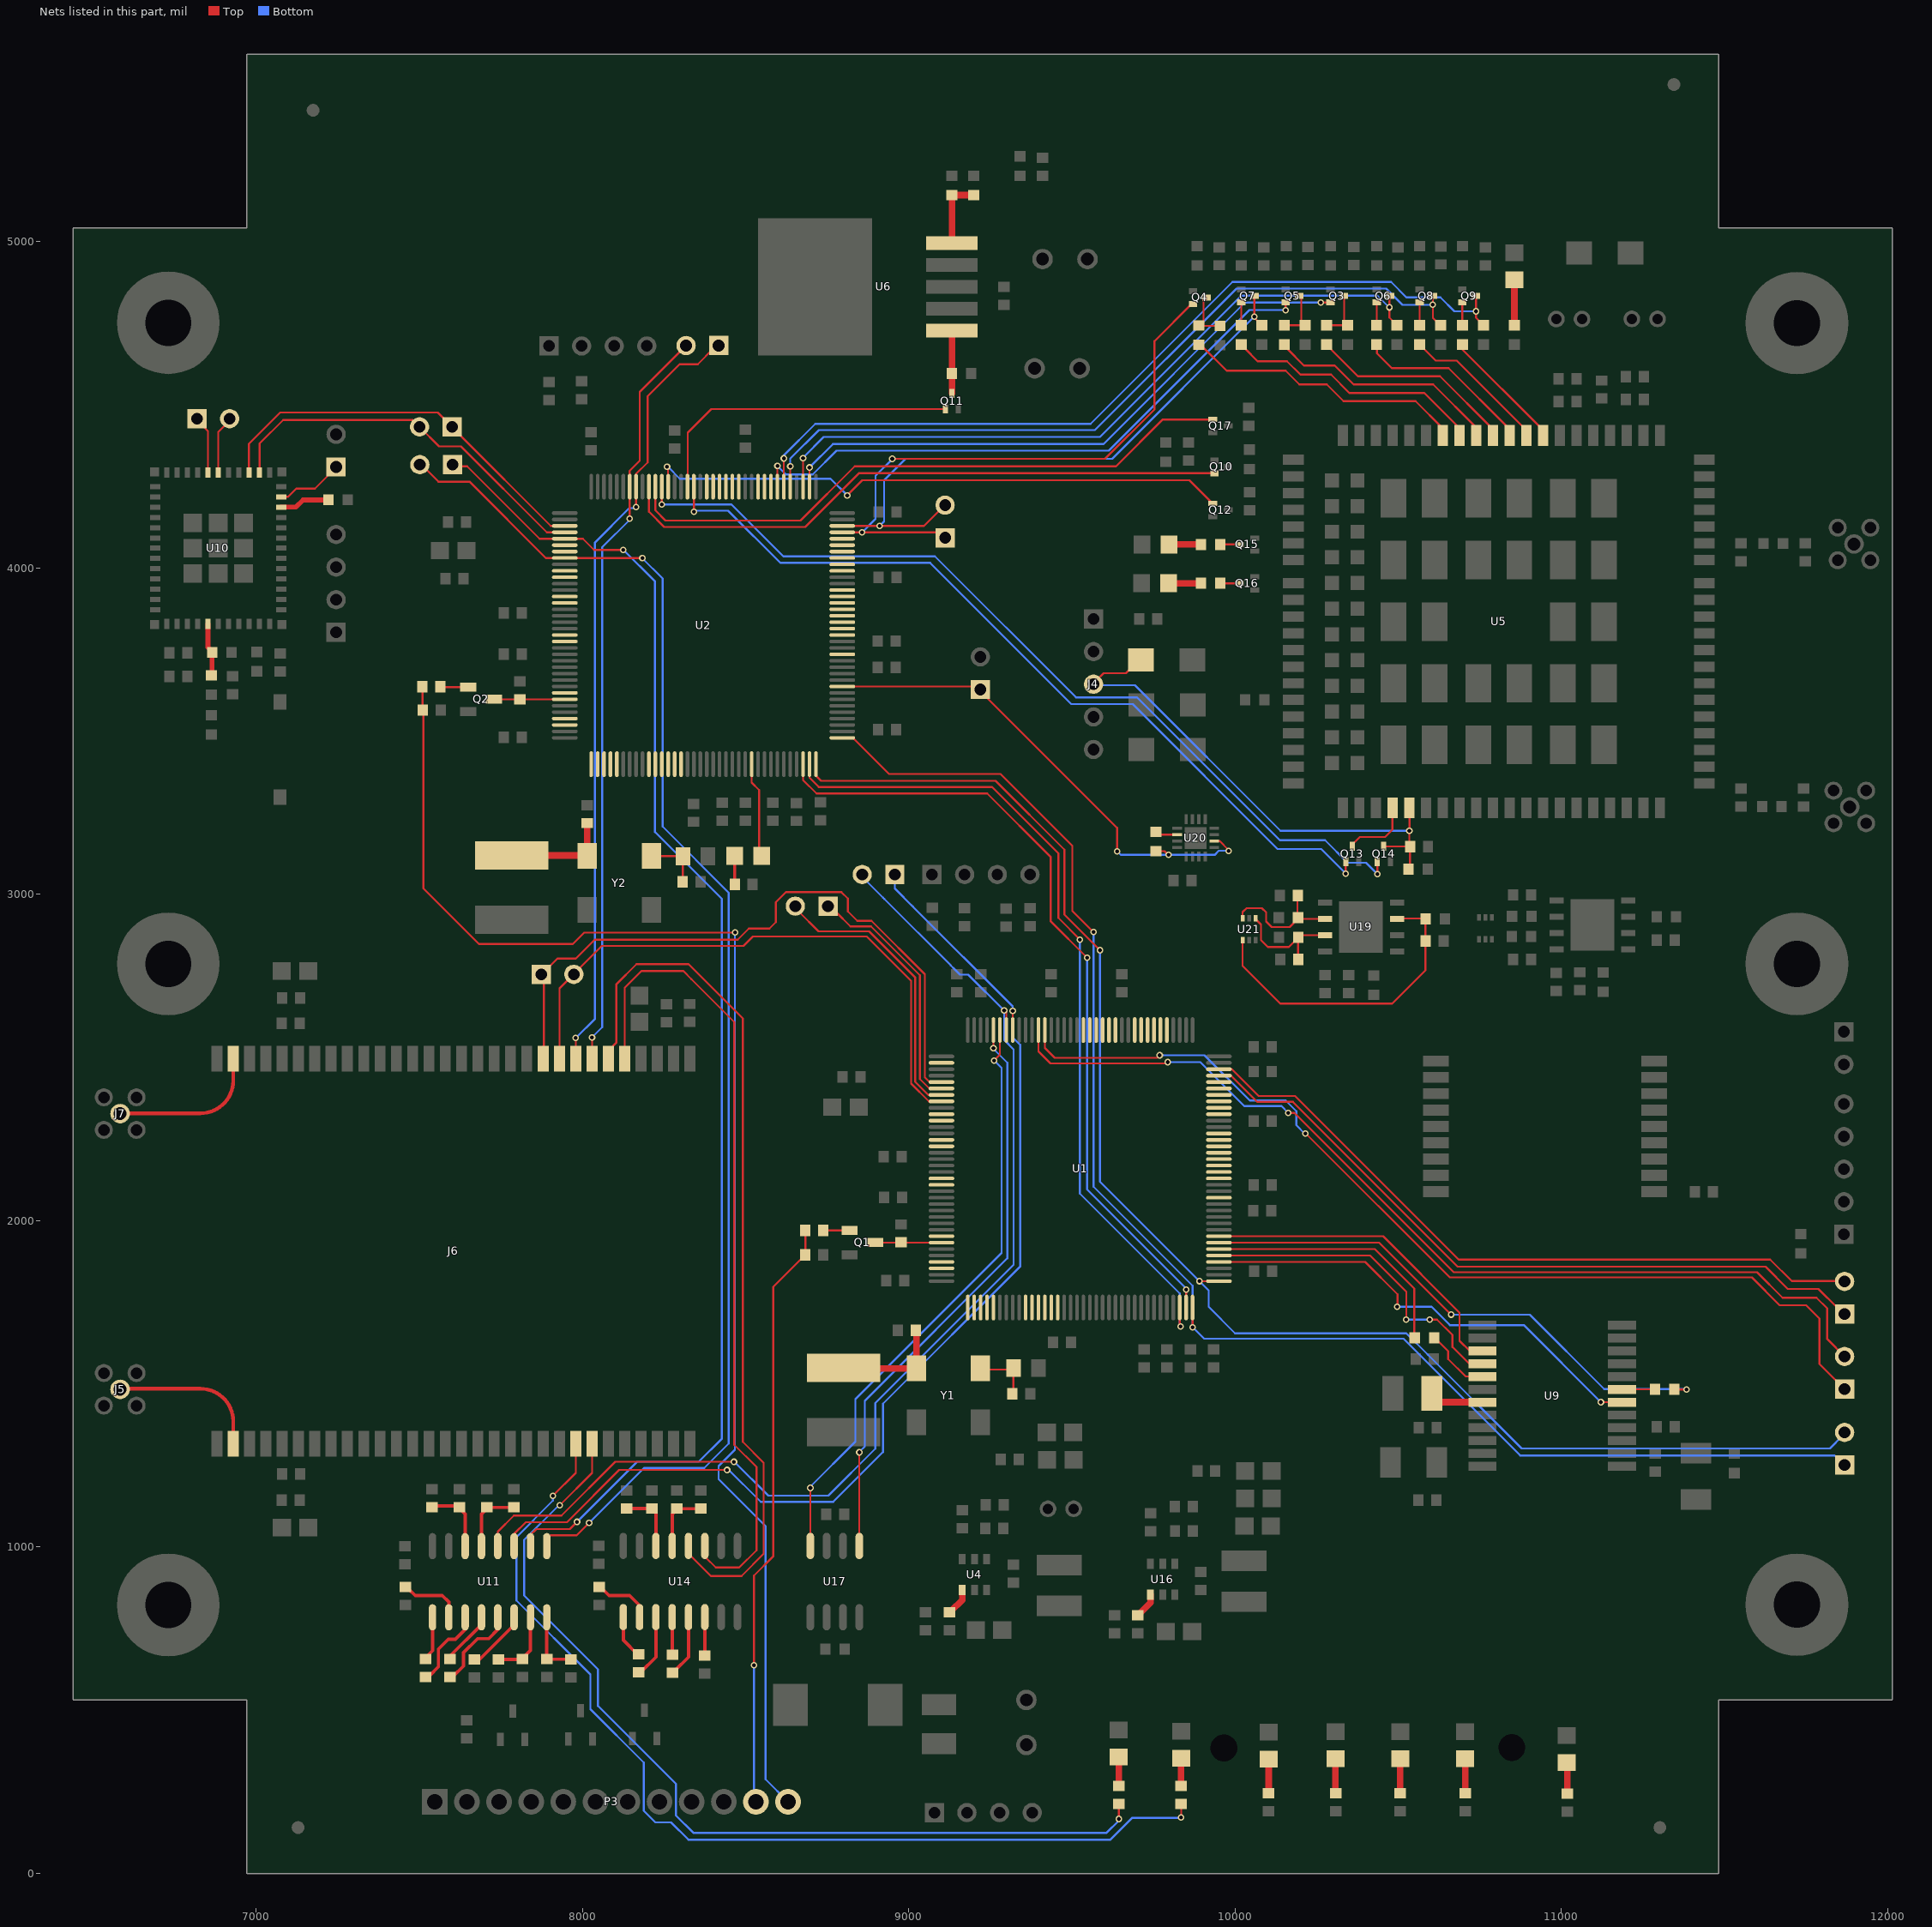
[diagram p0: the nets of this part, all layers, seen from the top]
# Altium PCB MISC86294.PcbDoc (part 6 of 8)
Units mil, origin at the board's own origin, x right, y up, seen from the top; angles counter-clockwise.
Board outline 5574.84 x 5574.84 mil, 4 copper layers (Top, GND02, PWR03, Bottom), stack 23.756 mil thick; 313 components, 311 nets, 1350 pads, 1701 vias.

## Via types
v1: diameter 20, hole 12, Top to Bottom, 1701 vias

## Nets (pads, with @x,y where several pads share a name; then routed paths per layer and width w, separated by ;. In a path a pad name is that pad's centre, name@x,y a point inside that pad or via, vN(x,y) a via of type N, cw(c..) or ccw(c..) an arc to the next point about the centre after c; other vN are vias at no path point) (continued)
NetC106_1: C106.1 U11.3 | length 235
  Top w10: C106.1@7532,607 7558,633 7558,687 7588,717 7610,717 7640.02,747.02 U11.3@7640.02,784.35
NetC106_2: C106.2 U11.1 | length 129.2
  Top w10: C106.2@7521,663 7540.02,682.02 U11.1@7540.02,784.35
NetC108_1: C108.1 U11.5 | length 255.2
  Top w10: C108.1@7605,605 7635,635 7635,676 7678,719 7712,719 7740.02,747.02 U11.5@7740.02,784.35
NetC108_2: C108.2 U11.4 | length 159.5
  Top w10: C108.2@7593,665 7690.02,762.02 U11.4@7690.02,784.35
NetC109_1: C109.1 U14.3 | length 187
  Top w10: C109.1@8179,617 8224.68,662.68 U14.3@8224.68,785.13
NetC109_2: C109.2 U14.1 | length 133.5
  Top w10: U14.1@8124.68,785.13 8124.68,714.32 C109.2@8169,670
NetC110_1: C110.1 U11.2 | length 186.2
  Top w10: C110.1@7467,871 7487,851 7570,851 7590.02,830.98 U11.2@7590.02,784.35
NetC112_1: C112.1 U14.2 | length 165.6
  Top w10: C112.1@8064,868 8081,851 8144,851 8174.68,820.32 U14.2@8174.68,785.13
NetC113_1: C113.1 U11.6 | length 185.3
  Top w10: C113.1@7672,655 7684,655 7790.02,761.02 U11.6@7790.02,784.35
NetC114_1: C114.1 U14.5 | length 180
  Top w10: C114.1@8284,622 8324.68,662.68 U14.5@8324.68,785.13
NetC114_2: C114.2 U14.4 | length 110.4
  Top w10: C114.2@8274.68,674.68 U14.4@8274.68,785.13
NetC115_2: C115.2 R75.2 U11.14 | length 206
  Top w10: C115.2@7543,1126 7615,1126 7640.02,1100.98 U11.14@7640.02,1002.38
NetC116_2: C116.2 R77.2 U11.13 | length 201.9
  Top w10: U11.13@7690.02,1002.38 7690.02,1101.02 7710,1121 C116.2@7785,1121
NetC117_1: C117.1 U14.6 | length 112.8
  Top w10: C117.1@8374.68,672.32 U14.6@8374.68,785.13
NetC118_2: C118.2 R76.2 U14.14 | length 200.9
  Top w10: C118.2@8133,1118 8215,1118 8224.68,1108.32 U14.14@8224.68,1003.16
NetC119_2: C119.2 R78.2 U14.13 | length 195.6
  Top w10: U14.13@8274.68,1003.16 8274.68,1100.68 8291,1117 C119.2@8366,1117
NetC120_1: C120.1 R81.2 U11.8 | length 194.2
  Top w10: U11.8@7890.02,784.35 7890.02,663.02 7897.03,656 C120.1@7960,656
NetC121_1: C121.1 R79.2 U11.7 | length 203
  Top w10: C121.1@7750,655 7812,655 7840.02,683.02 U11.7@7840.02,784.35
NetC123_1: C123.1 R82.2 U19.6 U21.3 | length 391.5
  Top w6: U21.3@10023,2928 10023,2946 10035,2958 10082,2958 10095,2945 10095,2917 10112,2900 10167,2900 10193,2926 R82.2@10193,2929 ; C123.1@10191,2990 10191,2934 10199.97,2925.03 U19.6@10275.59,2925.03
NetC129_1: C129.1 R80.2 U19.7 U21.1 | length 346.9
  Top w6: U21.1@10064,2921 U21.1@10065,2920 ; U21.1@10066,2921 10079,2908 10079,2860 10100,2839 10164.54,2839 R80.2@10193,2867.46 ; C129.1@10193,2812 R80.2@10193,2867.46 ; R80.2@10193.98,2868.45 R80.2@10193,2867.46 ; U19.7@10275.59,2875.03 10197.03,2875.03 10193,2871 R80.2@10193,2867.46
NetC130_1: C130.1 R90.2 U19.3 U21.4 | length 958
  Top w6: U21.4@10023,2861 10023,2781 10138.5,2665.5 10456.17,2665.5 10481.5,2665.5 10583.42,2767.42 C130.1@10583.42,2856.97 10583.42,2918.42 10575.84,2926 U19.3@10510,2926
NetC200_2: C200.2 R200.2 Y1.3 | length 193.7
  Top w6: Y1.3@9217.02,1543.84 R200.2@9324.84,1543.84 ; C200.2@9319.98,1456.16 R200.2@9319.98,1542.03
NetC201_1: C201.1 L200.1 Y1.4 | length 246.2
  Top w20: L200.1@8889,1548 8889.84,1547.16 9023.16,1547.16 C201.1@9023.16,1658.9
NetC202_2: C202.2 R201.2 Y2.3 | length 188.1
  Top w6: Y2.3@8211.06,3117.66 R201.2@8306.34,3117.66 ; C202.2@8306.89,3038.29 R201.2@8306.89,3124.11 ; C202.2@8308,3042 C202.2@8312.94,3037.06
NetC203_1: C203.1 L201.1 Y2.4 | length 318.5
  Top w20: L201.1@7782.37,3119.29 Y2.4@8010.29,3119.29 ; Y2.4@8014.05,3127.95 C203.1@8014.05,3218.57
NetD2_1: D2.1 R32.1 | length 74.9
  Top w20: R32.1@11017.89,244.25 D2.1@11017.89,319.11
NetD3_1: D3.1 R92.2 | length 78.6
  Top w20: R92.2@9834.65,267.73 D3.1@9834.65,346.35
NetD8_2: D8.2 R64.1 | length 131.5
  Top w20: R64.1@10856.07,4744.45 D8.2@10856.07,4875.93
NetD9_2: D9.2 R65.1 | length 100.4
  Top w20: D9.2@9794.52,4072.48 R65.1@9894.96,4072.48
NetD10_2: D10.2 R66.1 | length 78.1
  Top w20: D10.2@9810.52,3953.48 R66.1@9888.59,3953.48
NetD11_1: D11.1 R93.2 | length 86.4
  Top w20: D11.1@9636,351 9643.65,343.35 R93.2@9643.65,267.73
NetD12_1: D12.1 R84.2 | length 77
  Top w10: R84.2@8466.14,3030.11 D12.1@8466.14,3107.14
NetD12_2: D12.2 U2.26 | length 291.6
  Top w6: U2.26@8518.25,3399.13 8518.25,3342.75 8541,3320 D12.2@8541,3117
NetD13_1: D13.1 R7.2 | length 99.1
  Top w20: R7.2@10307.52,251.48 D13.1@10307.52,350.59
NetD14_1: D14.1 R6.2 | length 97.3
  Top w20: R6.2@10103,253 D14.1@10103,350.3
NetD15_1: D15.1 R9.2 | length 101.6
  Top w20: R9.2@10505.96,249.04 D15.1@10505.96,350.59
NetD16_1: D16.1 R98.2 | length 101.5
  Top w20: R98.2@10705.04,249.04 D16.1@10705.04,350.59
NetJ5_1: J5.1 J6.2 | length 460.3
  Top w11.55: J5.1@6595,1485 6829.01,1485 cw(c6829.01,1385) 6929.01,1385 J6.2@6929.01,1315.83
NetJ6_23: J6.23 R92.1 | length 3113.3
  Top w6: v1(7909,1157) 7979.01,1227.01 J6.23@7979.01,1315.83 ; v1(9834.65,170.65) R92.1@9834.65,212.62
  Bottom w6: v1(7909,1157) 7909,1142 7797,1030 7797,836 8024,609 8024,503 8187.64,339.36 8187.64,191.36 8223,156 8271,156 8324,103 9618,103 9685,170 v1@9833,170
NetJ6_24: J6.24 R93.1 | length 2860.9
  Top w6: v1(7930,1128) 8029.01,1227.01 J6.24@8029.01,1315.83 ; v1(9643.65,166.35) R93.1@9643.65,212.62
  Bottom w6: v1@7927,1128 7820.5,1021.5 7820.5,851.5 8047,625 8047,513 8286,274 8286,177 8339,124 9606,124 v1@9644,162 ; v1@7928.5,1126.5 v1(7930,1128)
NetJ6_35: J6.35 U14.11 | length 2476.8
  Top w6: J6.35@8129.01,2496.94 8129.01,2696 8129,2714 8180,2765 8309,2765 8333.5,2740.5 8465,2609 8465,1313 8533,1245 8533,990 8480,937 8408,937 U14.11@8377,968
NetJ6_36: J6.36 U14.12 | length 2695.9
  Top w6: J6.36@8079.01,2496.94 J6.36@8079.01,2525 ; J6.36@8083,2525 8103,2545 8103,2724 8165,2786 8325,2786 8351,2760 8491,2620 8491,1322 8555,1258 8555,979 8487,911 8393,911 8324.68,979.32 U14.12@8324.68,1003.16
NetJ6_37: J6.37 J15.2 U2.102 | length 2283.8
  Top w6: J6.37@8029.01,2496.94 v1(8029.01,2560.99) ; v1(8144.23,4151.23) U2.102@8144.23,4249.52 8144.23,4298.23 8175,4329 8175,4540 J15.2@8305,4670
  Bottom w6: v1(8029.01,2560.99) v1@8030.51,2562.49 ; v1@8030,2563 8060,2593 8060,4064 v1@8144,4148
NetJ6_38: J6.38 J15.1 U2.101 | length 2391.5
  Top w6: J6.38@7979.01,2496.94 v1(7979.01,2559.99) ; v1(8163.92,4187.08) U2.101@8163.92,4249.52 8163.92,4288.92 8199,4324 8199,4527 8297,4625 8353,4625 J15.1@8400,4672
  Bottom w6: v1(7979.01,2559.99) 8038,2618.97 8038,4009 8038,4079 8143,4184 v1@8164,4184
NetJ6_39: J6.39 J20.2 U1.116 | length 1845.6
  Top w6: J6.39@7929.01,2496.94 7929.01,2521 7929,2712 8059,2842 8215,2842 8493,2842 8522,2871 8871,2871 9007,2735 9007,2420 9061.31,2365.69 U1.116@9099.8,2365.69
NetJ6_40: J6.40 J20.1 U1.113 | length 2044.4
  Top w6: J6.40@7880,2521 J6.40@7880,2536 ; J20.1@7880,2760 7923,2803 7979,2803 8037,2861 8197,2861 8475,2861 8509.5,2895.5 8572.5,2895.5 8592,2915 8592,2976 8623,3007 8793,3007 8813,2987 8813,2948 8842,2919 8885,2919 9049,2755 9049,2439 9063.25,2424.75 U1.113@9099.8,2424.75 ; J6.40@7881,2536 7881,2755 7881,2757 J20.1@7882,2758
NetJ6_59: J6.59 J7.1 | length 458
  Top w11.55: J7.1@6596,2329 6829.01,2329 ccw(c6829.01,2429) 6929.01,2429 J6.59@6929.01,2496.94
NetJ9_1: J9.1 U10.23 | length 175.5
  Top w6: U10.23@7075.91,4218.48 7097.48,4218.48 7122.5,4243.5 7179.5,4243.5 J9.1@7223,4287
NetJ10_1: J10.1 U10.31 | length 167.9
  Top w6: J10.1@6822,4449 6851.5,4419.5 U10.31@6851.5,4293.28
NetJ10_2: J10.2 U10.30 | length 164.7
  Top w6: U10.30@6883,4293.28 6883,4417 J10.2@6912,4446
NetJ12_1: J12.1 U1.114 | length 733.1
  Top w6: J12.1@8777,2946 8821,2902 8884,2902 9034,2752 9034,2434 9062.94,2405.06 U1.114@9099.8,2405.06
NetJ12_2: J12.2 U1.115 | length 861.3
  Top w6: J12.2@8662,2948 8723,2887 8878,2887 9019,2746 9019,2717 ; 9019,2720 9019,2717 ; U1.115@9099.8,2385.38 9059.62,2385.38 9019,2426 9019,2717
NetJ13_1: J13.1 U1.101 U11.11 | length 3517
  Top w6: U11.11@7790.02,1002.38 7790.02,1040.02 7826,1076 7952,1076 8112,1236 v1(8443,1236) ; U1.101@9318.31,2584.2 v1(9318.31,2643.31)
  Bottom w6: v1@8443,1241 8546,1138 8768,1138 8921,1291 8921,1439 9341,1859 9341,2539 9318.31,2561.69 v1(9318.31,2643.31) 9318.31,2656.69 9013,2962 ; J13.1@8957,3053 8957,3018 9013,2962 ; 9008,2967 9013,2962
NetJ13_2: J13.2 U1.102 U11.12 | length 3609.8
  Top w6: U11.12@7740.02,1002.38 7740.02,1047.02 7789,1096 7935,1096 8100,1261 v1@8463,1261 ; v1@8465,1259 v1@8463,1261 ; v1@8465,1261 v1(8464,1261) v1@8463,1261 ; v1(9292,2644) 9298.24,2644 9298.62,2643.62 U1.102@9298.62,2584.2
  Bottom w6: v1@8465,1261 8569,1157 8753,1157 8897,1301 8897,1441 9321,1865 9321,2525 9292,2554 v1(9292,2644) 9182,2754 9157,2754 9139.7,2771.3 9139.43,2771.3 9128.3,2782.43 9128.3,2782.7 8925,2986 ; J13.2@8848,3048 8863,3048 8925,2986 ; 8921,2990 8925,2986
NetJ14_1: J14.1 U1.36 U2.37 | length 4686.6
  Top w6: U2.37@8799,3479.84 U2.37@8795.81,3479.84 8828.16,3479.84 8939,3369 9281,3369 9501,3149 9501,2949 v1@9566.5,2883.5 ; v1(9869.49,1673.49) U1.36@9869.49,1733.8
  Bottom w6: 9566,2781 9566,2776 ; v1(9566,2885) 9566,2776 ; J14.1@11848,1269 11837,1280 10874,1280 10516,1638 9904.98,1638 v1(9869.49,1673.49) 9869.49,1800.51 9566,2104 9566,2776
NetJ14_2: J14.2 U1.37 U2.36 | length 4699.2
  Top w6: U2.36@8715.1,3399.13 8715.1,3363.9 8731,3348 8802,3348 ; 8824,3348 8802,3348 ; v1(9586,2829) 9477,2938 9477,3137 9266,3348 8802,3348 ; v1(9890.49,1814.51) U1.37@9950.2,1814.51
  Bottom w6: v1@9586,2826 9586,2119 v1(9890.49,1814.51) 9919,1786 9919,1736 10000,1655 10525,1655 10590,1590 ; 10593,1587 10590,1590 ; 11628,1302 11623,1302 ; J14.2@11860,1339 11823,1302 11623,1302 ; 10590,1590 10878,1302 11623,1302
NetJ16_1: J16.1 U1.69 | length 2226.6
  Top w6: U1.69@9950.2,2444.43 9987.57,2444.43 10068,2364 10177,2364 10519.5,2021.5 ; 10546,1995 10519.5,2021.5 ; J16.1@11845,1734 11788,1791 11694,1791 11626,1859 10682,1859 10519.5,2021.5
NetJ16_2: J16.2 U1.70 | length 2181.7
  Top w6: U1.70@9950.2,2464.12 9989.88,2464.12 10072,2382 10184,2382 10685,1881 11640,1881 11706,1815 J16.2@11863,1815
NetJ17_1: J17.1 Q4.1 U2.69 | length 1809.5
  Top w6: U2.69@8795.81,4109.76 v1(8856.76,4109.76) J17.1@9097.24,4109.76 ; v1(8949,4335) 9601,4335 9753,4487 9753,4696 9868,4811 Q4.1@9874,4811
  Bottom w6: v1(8856.76,4109.76) 8898,4151 8898,4283 v1@8949,4334 ; v1@8952,4331 v1@8952,4332
NetJ17_2: J17.2 Q7.3 R44.1 U2.70 | length 1900.5
  Top w6: U2.70@8795.81,4129.44 v1(8910.44,4129.44) 9046.44,4129.44 J17.2@9096,4179 ; v1@10059,4767.55 R44.1@10082.1,4744.45 ; v1(10059,4771) Q7.3@10059,4830
  Bottom w6: v1(8910.44,4129.44) 8924,4143 8924,4269 8990,4335 9623,4335 v1(10059,4771)
NetJ19_1: J19.1 U2.111 U10.27 | length 1235.4
  Top w6: U10.27@6977,4298 6977,4381 7073,4477 7556,4477 J19.1@7600,4433 J19.1@7622.5,4410.5 ; J19.1@7622,4410 7902.56,4129.44 U2.111@7945.42,4129.44
NetJ19_2: J19.2 U2.112 U10.26 | length 1189.8
  Top w6: U10.26@7010,4300 7010,4382 7082,4454 7479,4454 J19.2@7500,4433 7560,4373 7627,4373 7890.24,4109.76 U2.112@7945.42,4109.76
NetJ21_1: J21.1 U2.113 U11.10 | length 4221.4
  Top w6: J21.1@7603,4312 7646,4312 7867.93,4090.07 U2.113@7945.42,4090.07 8000.93,4090.07 8035,4056 v1(8124,4056) ; U11.10@7840.02,1002.38 7840.02,1037.02 7858,1055 7961,1055 v1(7983,1077)
  Bottom w6: v1(7983,1077) 8167,1261 8356,1261 8427,1332 8427,2986 8222,3191 8222,3959 v1@8124,4057
NetJ21_2: J21.2 U2.116 U11.9 | length 4327.3
  Top w6: J21.2@7515,4308 7558,4265 7653,4265 7886.98,4031.02 U2.116@7945.42,4031.02 v1(8183.02,4031.02) ; U11.9@7890.02,1002.38 7890.02,1024.02 7902,1036 7982,1036 v1(8020,1074)
  Bottom w6: v1(8020,1074) 8188,1242 8373,1242 8448,1317 8448,2909 ; v1@8181,4032 8245,3968 8245,3459 ; 8245,3470 8245,3459 ; 8448,2916 8448,2909 ; 8245,3459 8245,3208 8448,3005 8448,2909
NetJ22_1: J22.1 U1.96 | length 3051.9
  Top w6: U1.96@9416.73,2584.2 9416.73,2529.27 9447,2499 9761,2499 v1(9769,2507) ; v1@10215.5,2268.5 10658,1826 11584,1826 11669,1741 11750,1741 11791,1700 11791,1561 J22.1@11868,1484
  Bottom w6: v1(9769,2507) 9906,2507 10045,2368 10155,2368 10187.5,2335.5 10187.5,2292.5 v1@10214,2266
  other v1: 10215,2267
NetJ22_2: J22.2 U1.97 | length 2981.2
  Top w6: U1.97@9397.05,2584.2 9397.05,2518.95 9434,2482 v1@9789,2482 ; v1@10158,2330 v1(10163,2330) 10182,2330 10670,1842 11600,1842 11678,1764 11782,1764 11815,1731 11815,1637 J22.2@11868,1584
  Bottom w6: v1(9793,2486) 9893,2486 10028,2351 10142,2351 v1(10163,2330)
NetJ23_1: J23.1 R91.1 U2.45 U20.2 | length 1563.6
  Top w6: U2.45@8795.81,3637.32 9204.68,3637.32 9638,3204 v1(9638,3132) ; R91.1@9756.87,3132.36 9783.64,3132.36 v1@9795,3121 ; U20.2@9936.24,3163.25 9952.75,3163.25 v1@9979,3137 ; v1(9980,3133) 9980,3128 9981,3128 9981,3138 v1@9980.5,3138.5
  Bottom w6: v1@9638,3133 9650,3121 v1(9796,3121) 9937,3121 9950,3134 v1@9979,3134 ; v1@9979,3132 9978,3131 9980,3131 v1(9980,3133)
NetL2_2: L2.2 U9.7 | length 128.8
  Top w20: L2.2@10629.27,1443.73 U9.7@10758.02,1443.73
NetP3_11: P3.11 R1.1 R2.2 | length 1784
  Top w6: v1(8525,638) 8525,912 8584,971 8584,1796.39 R1.1@8682.5,1894.89 ; R1.1@8682.89,1904.11 R2.2@8682.89,1970
  Bottom w6: P3.11@8525,242 v1(8525,638)
NetP3_12: P3.12 R13.1 R14.2 | length 4420.5
  Top w6: R13.1@7509.14,3575.14 R14.2@7509.14,3635.95 ; R13.1@7512,3562 7512,3018 7682,2848 7970,2848 8005,2883 v1(8467,2883)
  Bottom w6: v1@8467,2886 v1(8467,2883) 8467,1298 8417,1248 8417,1208 8561,1064 8561,287.76 P3.12@8629.71,219.05
NetQ1_1: Q1.1 R2.1 | length 73.2
  Top w6: R2.1@8745.4,1970.4 Q1.1@8818.63,1970.4
NetQ1_3: Q1.3 R3.2 U1.138 | length 194.2
  Top w6: Q1.3@8905.62,1932.62 U1.138@9099.8,1932.62
NetQ2_1: Q2.1 R14.1 | length 77.1
  Top w6: R14.1@7572.32,3635.32 Q2.1@7649.44,3635.32
NetQ2_3: Q2.3 R16.2 U2.138 | length 208.5
  Top w6: Q2.3@7736.95,3597.95 U2.138@7945.42,3597.95
NetQ3_1: Q3.1 U2.74 | length 1862.4
  Top w6: U2.74@8695.42,4249.52 v1(8695.42,4308.59) ; v1(10263,4814) 10288,4814 Q3.1@10289,4813
  Bottom w6: v1(8695.42,4308.59) 8766.83,4380 9596,4380 10030,4814 v1(10263,4814)
NetQ3_3: Q3.3 R37.2 R41.1 | length 144.7
  Top w6: R41.1@10280.6,4744.45 R37.2@10333.45,4744.45 ; Q3.3@10334,4832 10334,4754.95 R37.2@10344.5,4744.45
NetQ4_3: Q4.3 R39.2 R53.1 | length 142.4
  Top w6: R53.1@9896.45,4742.45 R39.2@9953.8,4742.45 ; R53.1@9903,4748 9903,4825 9903,4826 Q4.3@9908,4831
NetQ5_1: Q5.1 U2.79 | length 1864.2
  Top w6: U2.79@8596.99,4249.52 v1(8596.99,4312.99) ; v1(10154.78,4790.22) Q5.1@10154.78,4814.45
  Bottom w6: v1(8596.99,4312.99) 8622.98,4287 8705,4287 8778,4360 9613,4360 10044,4791 v1@10154,4791
NetQ5_3: Q5.3 R40.2 R48.1 | length 142.2
  Top w6: R48.1@10161.55,4744.45 R40.2@10214.45,4744.45 10203,4755.9 Q5.3@10203,4829
NetQ6_1: Q6.1 R43.1 | length 63.2
  Top w6: R43.1@10434.24,4751.24 Q6.1@10434.24,4814.45
NetQ6_3: Q6.3 R42.1 U2.75 | length 2202.6
  Top w6: U2.75@8675.73,4249.52 v1(8675.73,4336.73) ; Q6.3@10473,4832 v1(10473,4799) 10473,4767.75 R42.1@10496.3,4744.45
  Bottom w6: v1(8675.73,4336.73) v1@8678,4336.73 ; v1@8678,4341 8739,4402 9586,4402 10019,4835 10436,4835 10473,4798 v1(10473,4799)
NetQ7_1: Q7.1 R51.1 | length 64.8
  Top w6: R51.1@10018.62,4749.62 Q7.1@10018.62,4814.45
NetQ8_1: Q8.1 R47.1 | length 60
  Top w6: R47.1@10565.41,4754.41 Q8.1@10565.41,4814.45
NetQ8_3: Q8.3 R52.1 U2.77 | length 2388.1
  Top w6: U2.77@8636.36,4249.52 v1(8636.36,4311.64) ; Q8.3@10606,4830 v1(10606,4807) 10606,4767 10628.55,4744.45 R52.1@10630.09,4744.45
  Bottom w6: v1(8636.36,4311.64) 8636.36,4335.36 8724,4423 9570,4423 10004,4857 10463,4857 10513,4807 v1@10604,4807 ; v1@10605,4808 v1(10606,4807)
NetQ9_1: Q9.1 R50.1 | length 66
  Top w6: R50.1@10696.59,4748.41 Q9.1@10696.59,4814.45
NetQ9_3: Q9.3 R55.1 U2.78 | length 2570.9
  Top w6: U2.78@8616.67,4249.52 v1(8616.67,4336.32) ; Q9.3@10738,4831 v1(10738,4787) 10738,4767.34 R55.1@10760.89,4744.45
  Bottom w6: v1(8616.67,4336.32) 8616.67,4345.68 8713,4442 9557,4442 9992,4877 10478,4877 10525,4830 10629,4830 10672,4787 v1(10738,4787)
NetQ10_1: Q10.1 U2.99 | length 1865.5
  Top w6: U2.99@8203,4217 8203,4173 8250,4126 8682,4126 8846.6,4290.6 Q10.1@9936.82,4290.6
NetQ11_1: Q11.1 U2.93 | length 980.2
  Top w6: U2.93@8322,4255 8322,4415 8394.7,4487.7 Q11.1@9112.04,4487.7
NetQ11_3: Q11.3 R59.1 U6.1 | length 183
  Top w20: Q11.3@9132.04,4534.95 U6.1@9132.04,4717.96
NetQ12_1: Q12.1 U2.96 | length 1798.2
  Top w6: v1(8259,4311) 8261,4311 8262,4310 U2.96@8262,4280 ; v1(8811,4223) 8857,4269 9859.98,4269 Q12.1@9930.93,4198.05 Q12.1@9922.95,4198.05
  Bottom w6: v1(8259,4311) 8261,4311 8298,4274 8760,4274 v1(8811,4223)
NetQ13_1: Q13.1 U2.92 | length 2569
  Top w6: v1(8341.08,4172.92) U2.92@8341.08,4249.52 ; v1(10338.92,3063.08) Q13.1@10338.92,3099.74
  Bottom w6: v1@8341,4176 8446,4176 8606,4016 9065,4016 9498,3583 9686,3583 10130,3139 10264,3139 v1@10337,3066
NetQ14_1: Q14.1 U2.97 | length 2748.1
  Top w6: v1(8242.66,4195.34) U2.97@8242.66,4249.52 ; v1(10435.68,3062.32) Q14.1@10435.68,3099.74
  Bottom w6: v1@8246,4195 8456,4195 8615,4036 9080,4036 9512,3604 9699,3604 10137,3166 10276,3166 10345,3097 10401,3097 v1@10434,3064
NetQ15_3: Q15.3 R65.2 | length 48
  Top w6: R65.2@9965.48,4072.48 Q15.3@10013.49,4072.48
NetQ16_3: Q16.3 R66.2 | length 58
  Top w6: R66.2@9955.48,3953.48 Q16.3@10013.49,3953.48
NetQ17_1: Q17.1 U2.98 | length 1893
  Top w6: U2.98@8223,4220 8223,4177 8254,4146 8668,4146 8834,4312 9635,4312 9778.6,4455.6 Q17.1@9931.93,4455.6
NetR23_1: R23.1 U1.43 | length 1656
  Top w6: U1.43@9950.2,1932.62 10441.38,1932.62 v1(10662,1712) v1@10662.5,1711.5 ; R23.1@11346.64,1482.87 v1(11383.13,1482.87)
  Bottom w6: v1(10662,1712) 10768,1712 10903,1712 11131,1484 v1@11380,1484 ; v1@11380,1482.87 v1(11383.13,1482.87)
NetR23_2: R23.2 U9.19 | length 90.9
  Top w6: U9.19@11185.98,1483.1 R23.2@11276.9,1483.1
NetR24_1: R24.1 U1.42 | length 788.9
  Top w6: U1.42@9950.2,1912.94 10428.06,1912.94 10549,1792 R24.1@10549,1652
NetR24_2: R24.2 U9.5 | length 199.3
  Top w6: R24.2@10619,1634 10653,1600 10653,1576 10706.53,1522.47 U9.5@10758.02,1522.47
NetR26_1: R26.1 U4.4 | length 77.7
  Top w20: R26.1@9130,804 9163.6,837.6 U4.4@9163.6,867.76
NetR30_1: R30.1 U16.4 | length 74.5
  Top w20: R30.1@9705,794 9740.6,829.6 U16.4@9740.6,853.76
NetR41_2: R41.2 U5.65 | length 624.8
  Top w6: R41.2@10288,4676 10376,4588 10628,4588 10790.28,4425.72 U5.65@10790.28,4406.86
NetR43_2: R43.2 U5.64 | length 538.4
  Top w6: R43.2@10435,4675 10435,4658 10480,4613 10654,4613 10841.46,4425.54 U5.64@10841.46,4406.86
NetR47_2: R47.2 U5.63 | length 434
  Top w6: R47.2@10578,4673 10615,4636 10679,4636 10892.64,4422.36 U5.63@10892.64,4406.86
NetR48_2: R48.2 U5.66 | length 705.8
  Top w6: R48.2@10158,4674 10211,4621 10305,4621 10363,4563 10607,4563 10739.1,4430.9 U5.66@10739.1,4406.86
NetR50_2: R50.2 U5.62 | length 377.3
  Top w6: R50.2@10690,4679 10690,4677 10943.82,4423.18 U5.62@10943.82,4406.86
NetR51_2: R51.2 U5.67 | length 782.6
  Top w6: R51.2@10029,4674 10069,4634 10159,4634 10200,4593 10294,4593 10350,4537 10580,4537 10687.92,4429.08 U5.67@10687.92,4406.86
NetR53_2: R53.2 U5.68 | length 864.8
  Top w6: R53.2@9897,4680 R53.2@9901,4676 ; R53.2@9902,4677 9974,4605 10155,4605 10197,4563 10281,4563 10332,4512 10553,4512 10636.74,4428.26 U5.68@10636.74,4406.86
NetR60_1: R60.1 R63.2 U6.5 | length 200
  Top w20: U6.5@9132.17,5006.17 R63.2@9132.17,5143.17 R60.1@9195.17,5143.17
NetR71_1: R71.1 R72.1 U10.5 | length 154.9
  Top w15: U10.5@6851.5,3828.72 6851.5,3757.5 6864,3745 R71.1@6864,3679
NetR74_2: R74.2 U10.22 | length 148.2
  Top w15: U10.22@7075.91,4186.98 7120.98,4186.98 7143,4209 R74.2@7215,4209
NetR91_2: R91.2 U20.10 | length 50.9
  Top w6: R91.2@9771.13,3182.87 U20.10@9822.07,3182.87
NetU1_1: U1.1
NetU1_2: U1.2
NetU1_3: U1.3
NetU1_4: U1.4
NetU1_5: U1.5
NetU1_10: U1.10
NetU1_11: U1.11
NetU1_12: U1.12
NetU1_13: U1.13
NetU1_14: U1.14
NetU1_15: U1.15
NetU1_34: U1.34 U2.35 | length 2569.4
  Top w6: U2.35@8695.42,3399.13 8695.42,3357.59 8724,3329 9255,3329 9458,3126 9458,2928 v1@9526,2860 ; U1.34@9830.12,1733.8 9830.12,1676.12 9830.24,1676 v1(9833,1676)
  Bottom w6: v1(9524,2861) 9524,2774 9524,2083 9830.12,1776.88 9830.12,1676.12 9830.24,1676 v1(9833,1676)
NetU1_35: U1.35 U2.34 | length 2461.2
  Top w6: U2.34@8675.73,3399.13 8675.73,3350.27 8717,3309 8782,3309 ; 8790,3309 8782,3309 ; v1@9545,2807 9435,2917 9435,3114 9240,3309 8782,3309 ; U1.35@9849.8,1733.8 v1(9849.8,1788.8)
  Bottom w6: v1(9546,2806) 9546,2096 v1@9849.8,1792.2
NetU1_40: U1.40 U9.18 | length 1433.9
  Top w6: U1.40@9950.2,1873.57 10398.43,1873.57 10498,1774 v1@10498,1737 ; v1(11121.27,1443.73) U9.18@11185.98,1443.73
  Bottom w6: v1(10496,1736) 10602,1736 10658,1680 10885,1680 v1@11119,1446
NetU1_41: U1.41 U9.4 | length 1018.6
  Top w6: U1.41@9950.2,1893.25 10413.75,1893.25 10525,1782 10525,1742 ; v1@10525,1700 10525,1742 ; 10525,1738 10525,1742 ; v1(10596,1697) 10619,1697 10666,1650 10666,1613 10717.16,1561.84 U9.4@10758.02,1561.84
  Bottom w6: v1(10524,1697) v1(10596,1697)
NetU1_44: U1.44 U9.3 | length 989.7
  Top w6: U1.44@9950.2,1952.31 10453.69,1952.31 10688,1718 10688,1632 10719,1601 U9.3@10744,1601
NetU1_50: U1.50
NetU1_53: U1.53
NetU1_54: U1.54
NetU1_55: U1.55
NetU1_56: U1.56
NetU1_57: U1.57
NetU1_58: U1.58
NetU1_59: U1.59
NetU1_60: U1.60
NetU1_63: U1.63
NetU1_64: U1.64
NetU1_65: U1.65
NetU1_66: U1.66
NetU1_67: U1.67
NetU1_68: U1.68
NetU1_77: U1.77
NetU1_78: U1.78
NetU1_79: U1.79
NetU1_80: U1.80
NetU1_81: U1.81
NetU1_82: U1.82
NetU1_85: U1.85
NetU1_86: U1.86
NetU1_87: U1.87
NetU1_88: U1.88
NetU1_89: U1.89
NetU1_90: U1.90
NetU1_103: U1.103 U17.4 | length 1841.7
  Top w6: U17.4@8698,1003 v1(8698,1181) ; v1(9261,2491) 9278.94,2508.94 U1.103@9278.94,2584.2
  Bottom w6: v1@8696,1181 v1(8698,1181) ; v1@8696,1183 8836,1323 8836,1453 9284,1901 9284,2468 v1(9261,2491)
NetU1_104: U1.104 U17.1 | length 1780.2
  Top w6: U17.1@8848,1003 v1(8848,1290) ; v1(9259.25,2528.25) U1.104@9259.25,2584.2
  Bottom w6: v1@8850,1293 8864.72,1307.72 8864.72,1447.72 9302,1885 9302,2484 v1@9261,2525 ; v1@9260,2528 v1@9261,2528
NetU1_110: U1.110
NetU1_118: U1.118
NetU1_119: U1.119
NetU1_122: U1.122
NetU1_123: U1.123
NetU1_128: U1.128
NetU1_129: U1.129
NetU1_137: U1.137
NetU1_141: U1.141
NetU1_142: U1.142
NetU2_1: U2.1
NetU2_2: U2.2
NetU2_3: U2.3
NetU2_4: U2.4
NetU2_5: U2.5
NetU2_10: U2.10
NetU2_11: U2.11
NetU2_12: U2.12
NetU2_13: U2.13
NetU2_14: U2.14
NetU2_15: U2.15
NetU2_50: U2.50
NetU2_53: U2.53
NetU2_54: U2.54
NetU2_55: U2.55
NetU2_56: U2.56
NetU2_57: U2.57
NetU2_58: U2.58
NetU2_59: U2.59
NetU2_60: U2.60
NetU2_63: U2.63
NetU2_64: U2.64
NetU2_65: U2.65
NetU2_66: U2.66
NetU2_67: U2.67
NetU2_68: U2.68
NetU2_80: U2.80
NetU2_81: U2.81
NetU2_82: U2.82
NetU2_85: U2.85
NetU2_86: U2.86
NetU2_87: U2.87
NetU2_88: U2.88
NetU2_89: U2.89
NetU2_90: U2.90
NetU2_114: U2.114
NetU2_115: U2.115
NetU2_118: U2.118
NetU2_119: U2.119
NetU2_122: U2.122
NetU2_123: U2.123
NetU2_128: U2.128
NetU2_129: U2.129
NetU2_137: U2.137
NetU2_141: U2.141
NetU2_142: U2.142
PWRKEY: C79.1 D5.2 J4.3 Q14.3 R85.1 U5.21 | length 1557.9
  Top w6: J4.3@9575,3656 9597,3678 9665,3678 D5.2@9687,3700 ; D5.2@9690.12,3696.88 D5.2@9711.31,3718.07 ; Q14.3@10455.68,3146.98 10530.98,3146.98 10534,3150 v1@10534,3192 ; v1(10534,3195) 10534.37,3195 U5.21@10534.37,3265.13 ; R85.1@10536.02,3085.02 C79.1@10536.02,3146.93
  Bottom w6: J4.3@9575,3641 9693,3641 10139,3195 v1(10534,3195)
RESET_N: Q13.3 U5.20 | length 198.7
  Top w6: Q13.3@10358.92,3146.98 10358.92,3152.92 10382,3176 10460,3176 10482,3198 U5.20@10482,3249